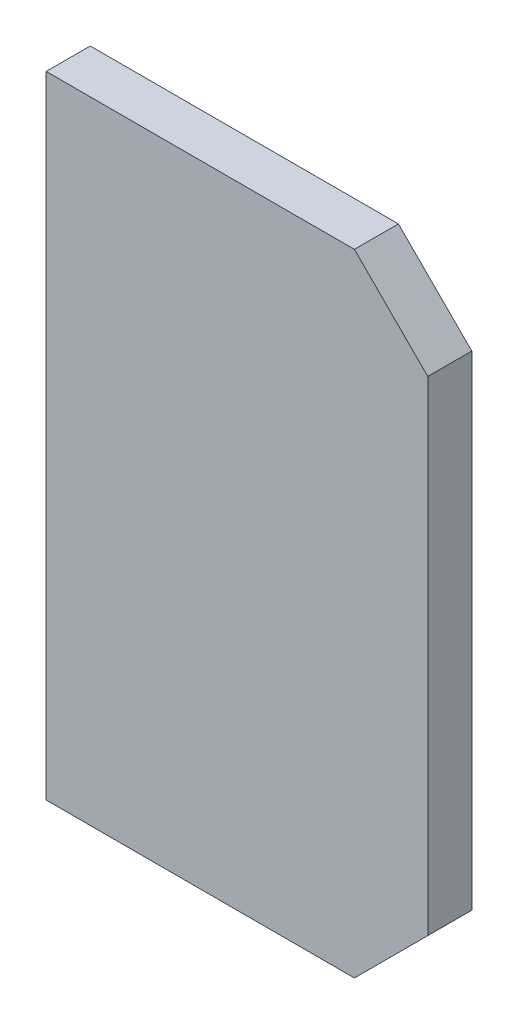
SolidWorks part; units mm, degrees
ref_plane "前视基准面" through (0, 0, 0) normal (0, 0, 1) x (1, 0, 0)
ref_plane "上视基准面" through (0, 0, 0) normal (0, 1, 0) x (1, 0, 0)
ref_plane "右视基准面" through (0, 0, 0) normal (1, 0, 0) x (0, 0, -1)
sketch "草图1" plane through (0, 0, 0) normal (0, 0, 1) x (1, 0, 0)
  line L0 (0, 0) -> (26, 0)
  line L1 (26, 0) -> (26, 43)
  line L2 (26, 43) -> (0, 43)
  line L3 (0, 43) -> (0, 0)
  dimension "D1" = 26
  dimension "D2" = 43
extrude "凸台-拉伸1" add sketch "草图1" along normal blind 3
chamfer "倒角1" distance 5 angle 45 2 edges at (26, 0, 1.5) (26, 43, 1.5)
